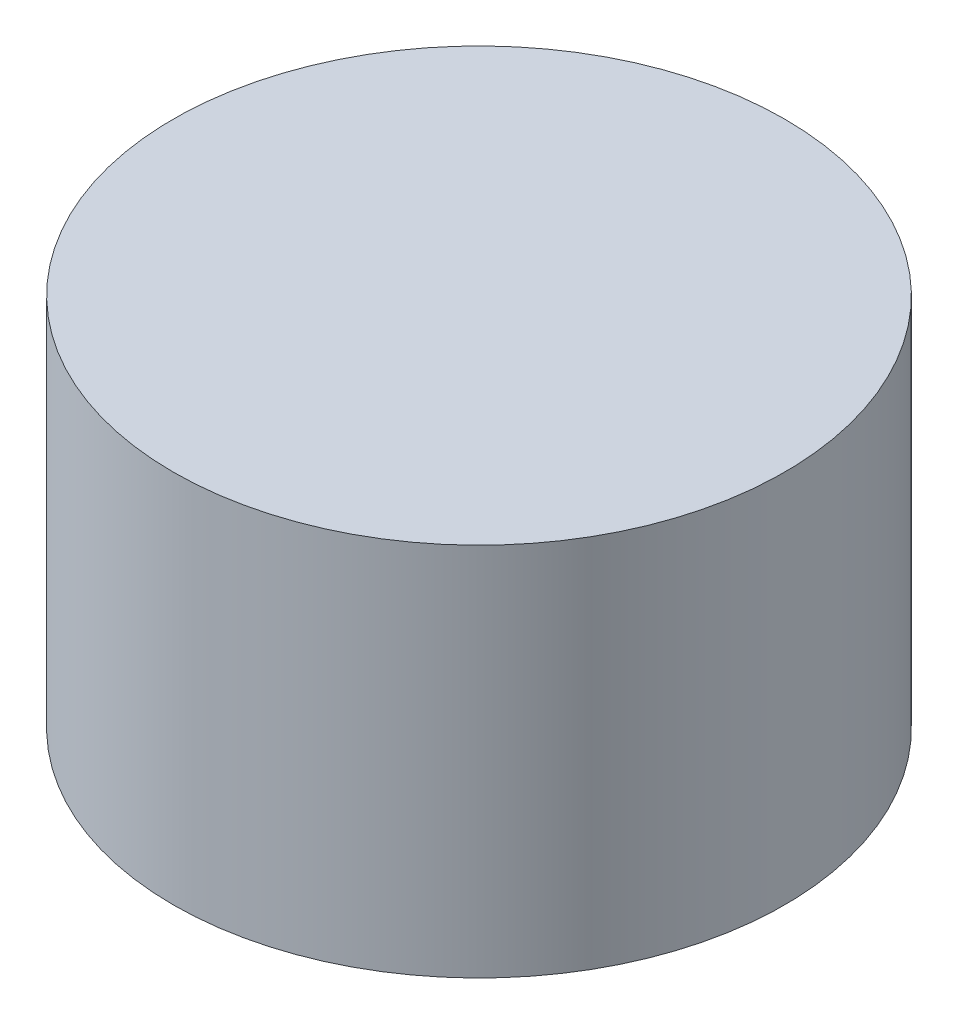
from build123d import *

# Parameters (mm, degrees)
SKETCH_1_R      = 24.470155971
EXTRUDE_1_DEPTH = 30


with BuildPart() as part:
    # 草图1 → 凸台-拉伸1 (new body)
    with BuildSketch(Plane(origin=(0, 0, 0), x_dir=(1, 0, 0), z_dir=(0, 1, 0))):
        with Locations(Location((0, 0, 0), (0, 0, 270))):
            Circle(SKETCH_1_R)
    extrude(amount=EXTRUDE_1_DEPTH)


solid = part.part
